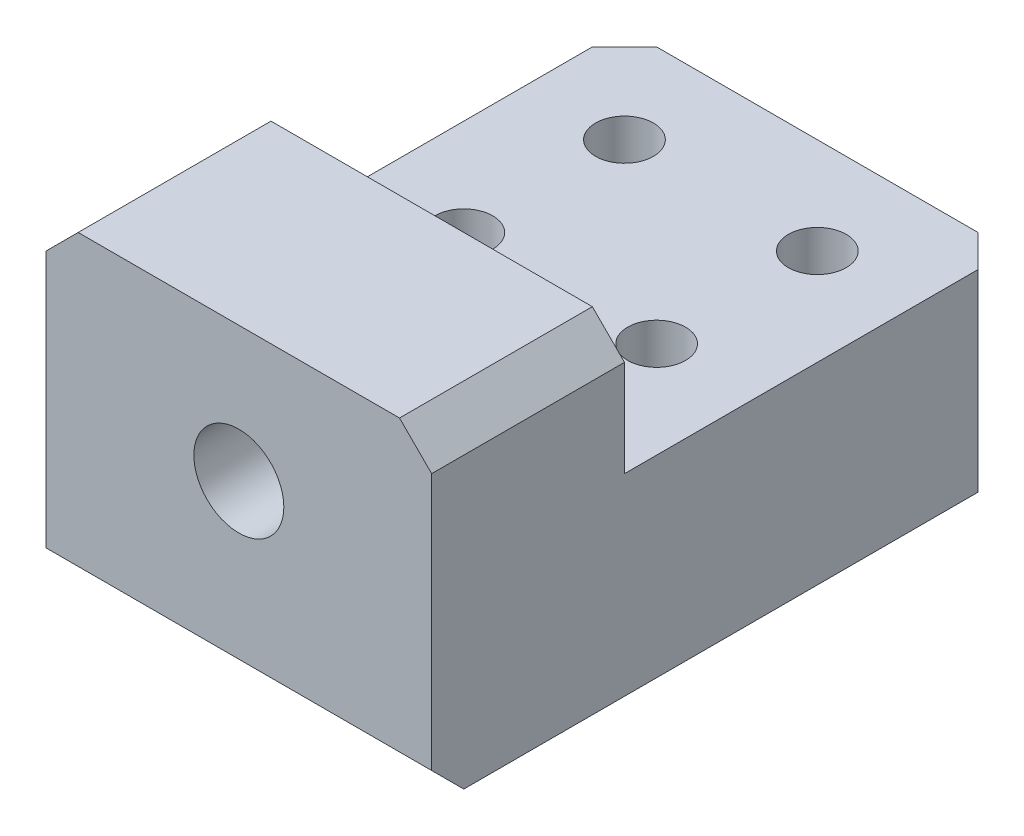
SolidWorks part; units mm, degrees
ref_plane "前视" through (0, 0, 0) normal (0, 0, 1) x (1, 0, 0)
ref_plane "上视" through (0, 0, 0) normal (0, 1, 0) x (1, 0, 0)
ref_plane "右视" through (0, 0, 0) normal (1, 0, 0) x (0, 0, -1)
sketch "草图1" plane through (0, 0, 0) normal (0, 0, 1) x (1, 0, 0)
  line L1 (-30, 15) -> (30, 15)
  line L2 (-30, 15) -> (-30, -15)
  line L3 (-30, -15) -> (30, -15)
  line L4 (30, 15) -> (30, -15)
  line L5 (-30, 15) -> (30, -15) construction
  line L6 (-30, -15) -> (30, 15) construction
  point P0 (0, 0)
  dimension "D1" = 60
  dimension "D2" = 30
extrude "凸台-拉伸1" add sketch "草图1" along normal blind 90
sketch "草图2" plane through (0, 15, 0) normal (0, 1, 0) x (1, 0, 0)
  line L0 (30, -90) -> (30, 0) construction
  line L1 (-30, -90) -> (30, -90)
  line L2 (-30, -90) -> (-30, -60)
  line L3 (-30, -60) -> (30, -60)
  line L4 (30, -90) -> (30, -60)
  dimension "D1" = 30
extrude "凸台-拉伸2" add sketch "草图2" along normal blind 20
hole_wizard "Ø9.0 (9) 直径孔1" positions "草图3" profile "草图4" hole size "Ø9.0" standard "GB" end condition through all
sketch "草图3" plane through (0, 15, 0) normal (0, 1, 0) x (1, 0, 0)
  line L0 (0, 0) -> (0, -33.5041) construction
  line L2 (30, 0) -> (-30, 0) construction
  point P0 (-15, -15)
  point P2 (15, -15)
  point P4 (-15, -40)
  point P6 (15, -40)
  dimension "D1" = 30
  dimension "D2" = 15
  dimension "D3" = 25
sketch "草图4" plane through (-15, 15, 15) normal (1, 0, 0) x (0, 0, 1)
  line L0 (0, 0) -> (0, 30)
  line L1 (0, 30) -> (4.5, 30)
  line L2 (4.5, 30) -> (4.5, 0)
  line L5 (4.5, 0) -> (0, 0)
  line L11 (0, -6.35) -> (0, 107.95) construction
  dimension "通孔孔直径" = 9
  dimension "通孔孔深度" = 30
hole_wizard "M16 螺纹孔1" positions "草图5" profile "草图6" tap size "M16" standard "GB"
sketch "草图5" plane through (0, 0, 90) normal (0, 0, 1) x (1, 0, 0)
  line L0 (-30, 35) -> (30, 35) construction
  point P0 (0, 14)
  dimension "D1" = 21
sketch "草图6" plane through (0, 14, 90) normal (1, 0, 0) x (0, -1, 0)
  line L0 (0, 0) -> (0, 42.206)
  line L1 (0, 42.206) -> (7, 38)
  line L2 (7, 38) -> (7, 0)
  line L5 (7, 0) -> (0, 0)
  line L10 (0, 42.206) -> (-7, 38) construction
  line L11 (0, -6.35) -> (0, 107.95) construction
  dimension "螺纹孔钻头直径" = 14
  dimension "螺纹孔钻头深度" = 38
  dimension "导头角度" = 118
cosmetic thread "孔螺蚊线1" parameters "D1"=30, "D2"=16
chamfer "倒角1" distance 5 angle 45 4 edges at (-30, 0, 0) (30, 0, 0) (-30, 35, 75) (30, 35, 75)
chamfer "倒角2" distance 5 angle 45 1 edges at (0, -15, 90)
